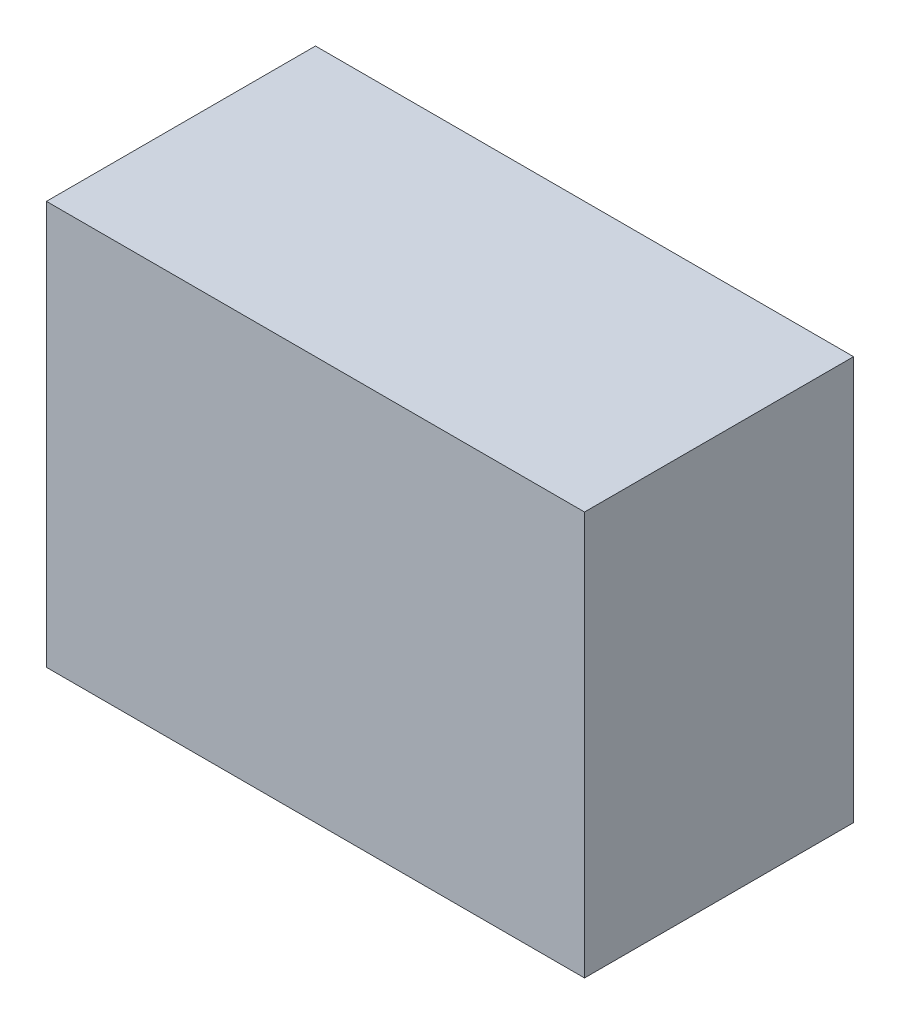
from build123d import *

# Parameters (mm, degrees)
SKETCH1_W           = 20
SKETCH1_H           = 10
BOSS_EXTRUDE1_DEPTH = 15


with BuildPart() as part:
    # Sketch1 → Boss-Extrude1 (new body)
    with BuildSketch(Plane(origin=(0, 0, 0), x_dir=(1, 0, 0), z_dir=(0, 1, 0))):
        with Locations((10, 5)):
            Rectangle(SKETCH1_W, SKETCH1_H)
    extrude(amount=BOSS_EXTRUDE1_DEPTH)


solid = part.part
